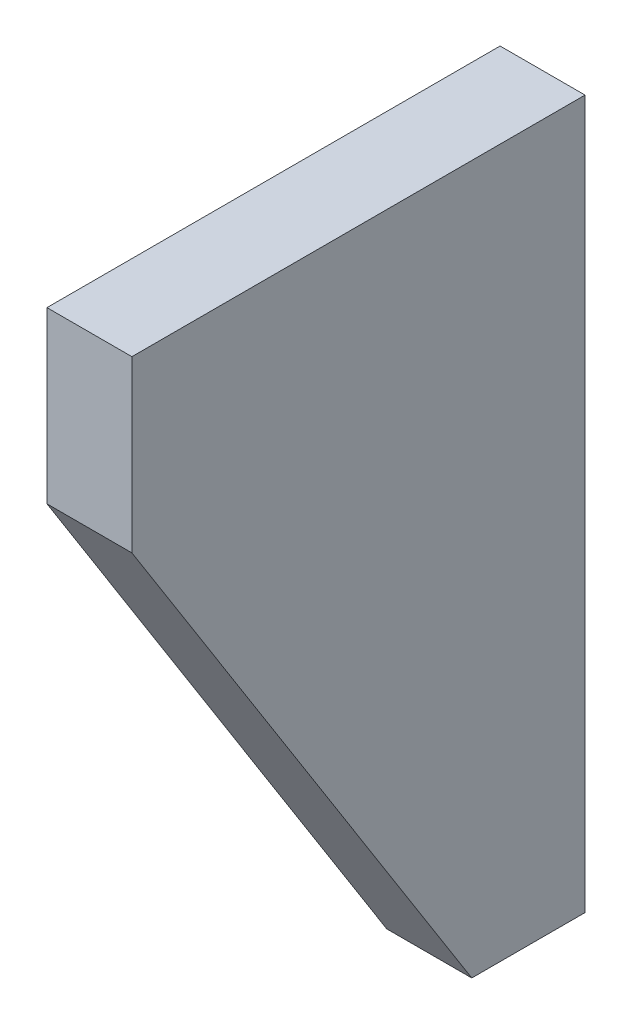
SolidWorks part; units mm, degrees
material "Q235-A"
ref_plane "Front Plane" through (0, 0, 0) normal (0, 0, 1) x (1, 0, 0)
ref_plane "Top Plane" through (0, 0, 0) normal (0, 1, 0) x (1, 0, 0)
ref_plane "Right Plane" through (0, 0, 0) normal (1, 0, 0) x (0, 0, -1)
sketch "Sketch1" plane through (0, 0, 0) normal (1, 0, 0) x (0, 0, -1)
  line L0 (0, 0) -> (0, 125)
  line L1 (0, 125) -> (-80, 125)
  line L2 (-80, 125) -> (-80, 95)
  line L3 (-80, 95) -> (-20, 0)
  line L4 (-20, 0) -> (0, 0)
  dimension "D1" = 20
  dimension "D2" = 30
  dimension "D3" = 80
  dimension "D4" = 125
extrude "Boss-Extrude1" add sketch "Sketch1" along normal mid plane 15
